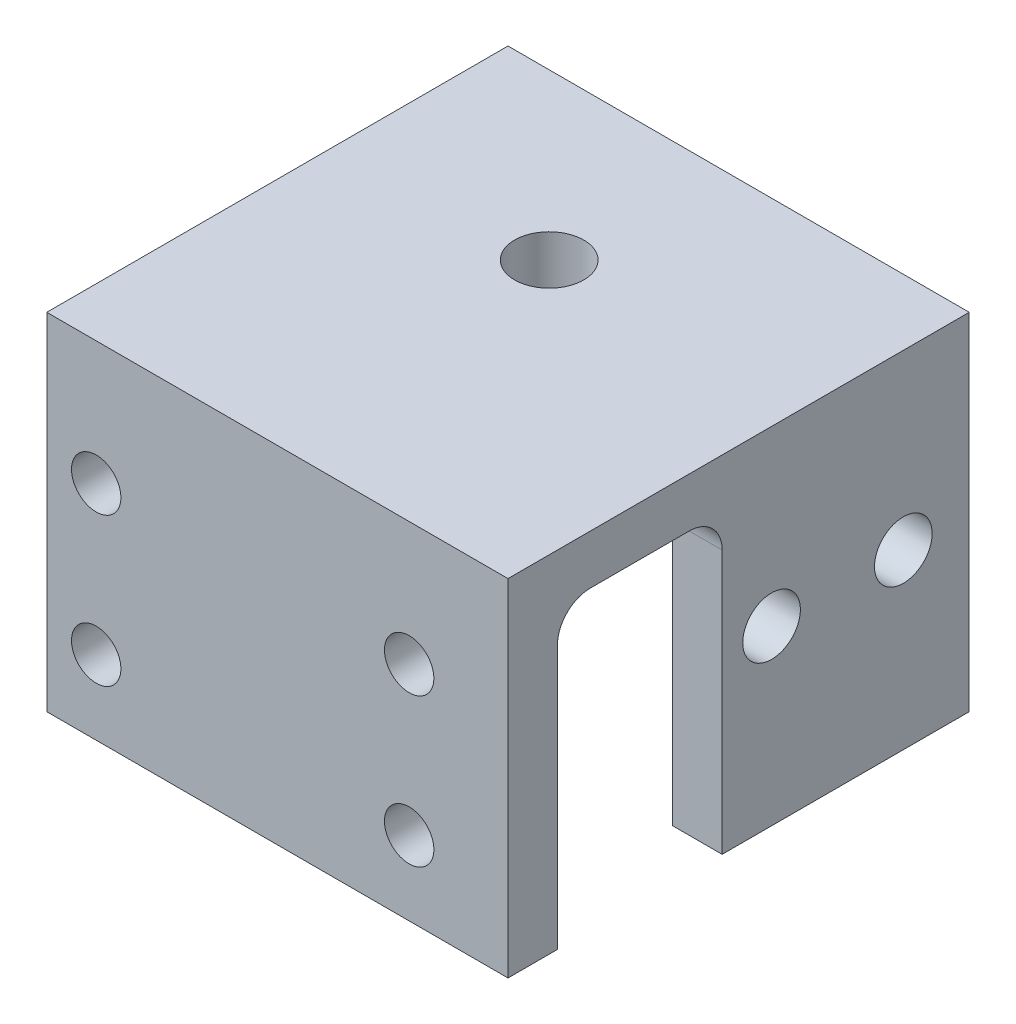
from build123d import *

# Parameters (mm, degrees)
SKETCH1_W           = 25
SKETCH1_H           = 18
SKETCH1_R           = 1.5
BOSS_EXTRUDE1_DEPTH = 3
SKETCH2_W           = 25
SKETCH2_H           = 28
SKETCH2_R           = 2.1
BOSS_EXTRUDE2_DEPTH = 3
SKETCH3_R           = 1.75
BOSS_EXTRUDE3_DEPTH = 3


with BuildPart() as part:
    # Sketch1 → Boss-Extrude1 (new body)
    with BuildSketch(Plane.XY):
        Rectangle(SKETCH1_W, SKETCH1_H)
        with Locations((-9.5, 4.5)):
            Circle(SKETCH1_R, mode=Mode.SUBTRACT)
        with Locations((9.5, 4.5)):
            Circle(SKETCH1_R, mode=Mode.SUBTRACT)
        with Locations((9.5, -4.5)):
            Circle(SKETCH1_R, mode=Mode.SUBTRACT)
        with Locations((-9.5, -4.5)):
            Circle(SKETCH1_R, mode=Mode.SUBTRACT)
    extrude(amount=BOSS_EXTRUDE1_DEPTH)

    # Sketch2 → Boss-Extrude2 (add)
    with BuildSketch(Plane(origin=(0, 9, 0), x_dir=(1, 0, 0), z_dir=(0, 1, 0))):
        with Locations((0, 11)):
            Rectangle(SKETCH2_W, SKETCH2_H)
        with Locations(Location((0, 15, 0), (0, 0, 270))):
            Circle(SKETCH2_R, mode=Mode.SUBTRACT)
    extrude(amount=BOSS_EXTRUDE2_DEPTH)

    # Sketch3 → Boss-Extrude3 (add)
    with BuildSketch(Plane.ZY.offset(-12.5)):
        with BuildLine():
            Line((0, -9), (0, 7))
            ThreePointArc((0, 7), (-0.585786438, 8.414213562), (-2, 9))
            Line((-2, 9), (-8, 9))
            ThreePointArc((-8, 9), (-9.414213562, 8.414213562), (-10, 7))
            Line((-10, 7), (-10, -9))
            Line((-10, -9), (-25, -9))
            Line((-25, -9), (-25, 12))
            Line((-25, 12), (3, 12))
            Line((3, 12), (3, -9))
            Line((3, -9), (0, -9))
        make_face()
        with Locations((-21, 1.5)):
            Circle(SKETCH3_R, mode=Mode.SUBTRACT)
        with Locations((-13, 1.5)):
            Circle(SKETCH3_R, mode=Mode.SUBTRACT)
    extrude(amount=-BOSS_EXTRUDE3_DEPTH)


solid = part.part
